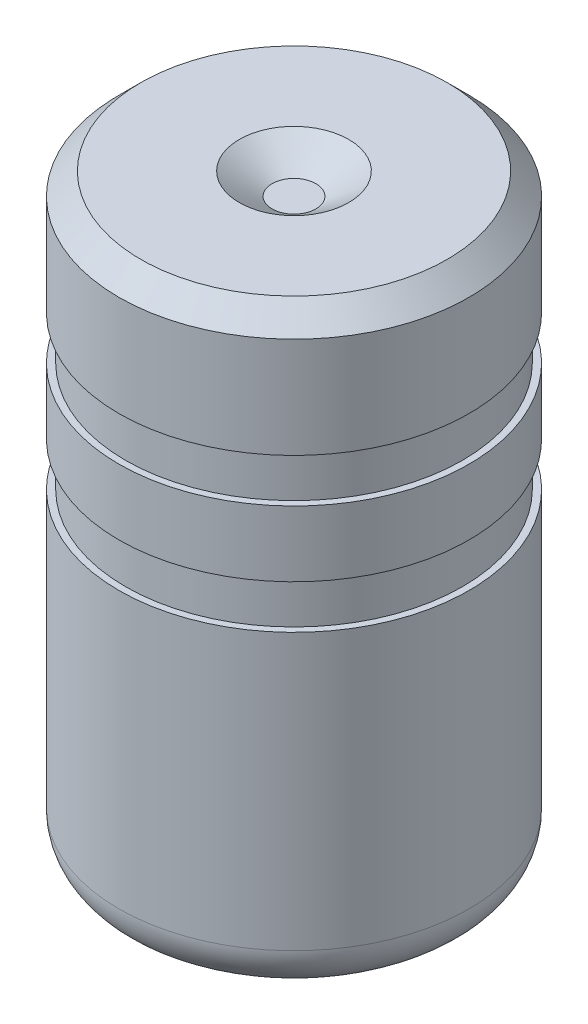
SolidWorks part; units mm, degrees
material "ABS"
ref_plane "前视基准面" through (0, 0, 0) normal (0, 0, 1) x (1, 0, 0)
ref_plane "上视基准面" through (0, 0, 0) normal (0, 1, 0) x (1, 0, 0)
ref_plane "右视基准面" through (0, 0, 0) normal (1, 0, 0) x (0, 0, -1)
sketch "草图1" plane through (0, 0, 0) normal (0, 0, 1) x (1, 0, 0)
  line L0 (0, 0) -> (0, 14.0736) construction
  line L1 (-3.25, 0) -> (-3.25, 12.5)
  line L2 (-3.85, 7.3) -> (-4, 7.3)
  line L3 (-4, 8.3) -> (-4, 9.8)
  line L4 (-4, 10.8) -> (-4, 13.1)
  line L10 (-1.25, 13.6) -> (-0.5, 13.1)
  line L11 (-3.25, 12.5) -> (0, 12.5)
  line L12 (-0.5, 13.1) -> (0, 13.1)
  line L13 (0, 12.5) -> (0, 13.1)
  line L15 (-4, 1) -> (-4, 7.3)
  line L16 (-3.5, 13.6) -> (-1.25, 13.6)
  line L17 (-4, 13.1) -> (-3.5, 13.6)
  line L18 (-3.85, 10.8) -> (-4, 10.8)
  line L19 (-3.85, 7.3) -> (-3.85, 8.3)
  line L20 (-3.85, 9.8) -> (-3.85, 10.8)
  line L21 (-4, 9.8) -> (-3.85, 9.8)
  line L22 (-3.85, 8.3) -> (-4, 8.3)
  arc A0 (-4, 1) -> (-3.25, 0) centre (-2.9583, 1) ccw
  point P19 (-4, 13.6)
  dimension "D9" = 1
  dimension "D1" = 6.5
  dimension "D2" = 1
  dimension "D3" = 1
  dimension "D4" = 7.7
  dimension "D5" = 7.3
  dimension "D7" = 1.5
  dimension "D8" = 8
  dimension "D10" = 13.6
  dimension "D11" = 0.5
  dimension "D12" = 12.5
  dimension "D14" = 1
  dimension "D15" = 2.5
revolve "旋转1" add sketch "草图1" angle 360 about L0
